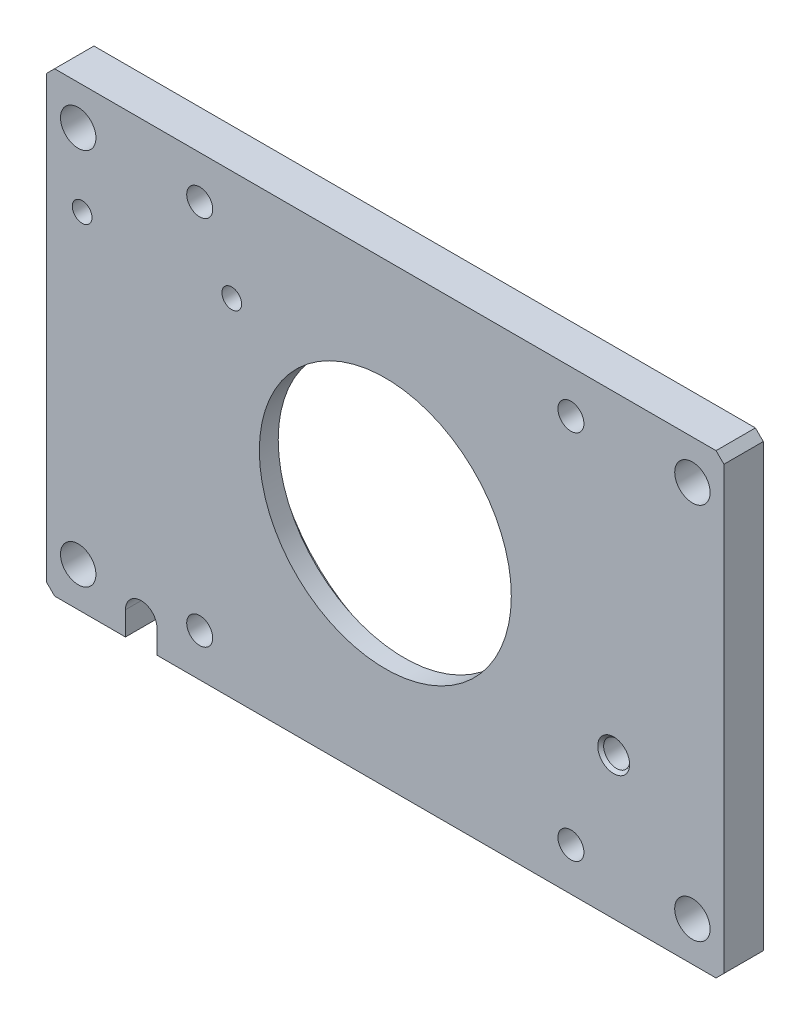
from build123d import *

# Parameters (mm, degrees)
SKETCH_1_W                   = 86
SKETCH_1_H                   = 58
SKETCH_1_R                   = 16
SKETCH_1_R_2                 = 2.25
EXTRUDE_1_DEPTH              = 5
HOLE_WIZARD_M3_1_D           = 2.5
HOLE_WIZARD_M4_1_D           = 3.3
MIRROR_2_COPY_1_D            = 3.3
CUT_EXTRUDE_1_DEPTH          = 53.820450585
CHAMFER_1_SIZE               = 1
SKETCH_10_W                  = 216.550460162
SKETCH_10_H                  = 17.046792279
CUT_EXTRUDE_4_DEPTH          = 73.374028491
SKETCH_11_R                  = 19.5
CUT_EXTRUDE_5_DEPTH          = 2.6
SKETCH_13_R                  = 1.350406535
CUT_EXTRUDE_6_DEPTH          = 10
HOLE_WIZARD_M4_3_D           = 3.3
HOLE_WIZARD_M4_3_DEPTH       = 11.5
HOLE_WIZARD_M4_3_CSINK_D     = 4.05
HOLE_WIZARD_M4_3_CSINK_ANGLE = 90
HOLE_WIZARD_M4_3_TIP         = 0.991420021


with BuildPart() as part:
    # 草图1 → 凸台-拉伸1 (new, symmetric)
    with BuildSketch(Plane.XY):
        Rectangle(SKETCH_1_W, SKETCH_1_H)
        Circle(SKETCH_1_R, mode=Mode.SUBTRACT)
        with Locations((-39, 24)):
            Circle(SKETCH_1_R_2, mode=Mode.SUBTRACT)
        with Locations(Location((39, 24, 0), (0, 0, 180))):
            Circle(SKETCH_1_R_2, mode=Mode.SUBTRACT)
        with Locations((39, -24)):
            Circle(SKETCH_1_R_2, mode=Mode.SUBTRACT)
        with Locations(Location((-39, -24, 0), (0, 0, 180))):
            Circle(SKETCH_1_R_2, mode=Mode.SUBTRACT)
    extrude(amount=EXTRUDE_1_DEPTH, both=True)

    # M3 螺纹孔1 (through all)
    with Locations(Plane.XY.offset(5)):
        with Locations((-38.5, 15), (-19.5, 15)):
            Hole(HOLE_WIZARD_M3_1_D / 2)

    # M4 螺纹孔1 (through all)
    with Locations(Plane.XY.offset(5)):
        with Locations((-23.57, 23.57)):
            hole_wizard_m4_1 = Hole(HOLE_WIZARD_M4_1_D / 2)

    # 镜向1: M4 螺纹孔1 across plane
    add(hole_wizard_m4_1.mirror(Plane.ZX), mode=Mode.SUBTRACT)

    # 镜向2: M4 螺纹孔1 across plane
    add(hole_wizard_m4_1.mirror(Plane(origin=(0, 0, 0), x_dir=(0, 0, 1), z_dir=(1, 0, 0))), mode=Mode.SUBTRACT)

    # 镜向2 copy 1 (through all)
    with Locations(Plane(origin=(0, 0, 5), x_dir=(-1, 0, 0), z_dir=(0, 0, 1))):
        with Locations((-23.57, 23.57)):
            Hole(MIRROR_2_COPY_1_D / 2)

    # 草图7 → 切除-拉伸1 (cut, through all)
    with BuildSketch(Plane.XY.offset(5)):
        with BuildLine():
            Line((-33, -29), (-33, -26))
            ThreePointArc((-33, -26), (-31, -24), (-29, -26))
            Line((-29, -26), (-29, -29))
            ThreePointArc((-29, -29), (-31, -31), (-33, -29))
        make_face()
    extrude(amount=-CUT_EXTRUDE_1_DEPTH, mode=Mode.SUBTRACT)

    # 倒角1
    chamfer_1_edges = [part.edges().sort_by_distance(p)[0] for p in [
        (43, -29, 0),
        (-43, -29, 0),
        (-43, 29, 0),
        (43, 29, 0),
    ]]
    chamfer(chamfer_1_edges, length=CHAMFER_1_SIZE)

    # 草图10 → 切除-拉伸4 (cut, through all)
    with BuildSketch(Plane(origin=(0, 29, 0), x_dir=(1, 0, 0), z_dir=(0, 1, 0))):
        with Locations((51.936518235, 8.52339614)):
            Rectangle(SKETCH_10_W, SKETCH_10_H)
    extrude(amount=-CUT_EXTRUDE_4_DEPTH, mode=Mode.SUBTRACT)

    # 草图11 → 切除-拉伸5 (cut)
    with BuildSketch(Plane(origin=(0, 0, 0), x_dir=(-1, 0, 0), z_dir=(0, 0, -1))):
        Circle(SKETCH_11_R)
    extrude(amount=-CUT_EXTRUDE_5_DEPTH, mode=Mode.SUBTRACT)

    # 草图13 → 切除-拉伸6 (cut)
    with BuildSketch(Plane.XY.offset(5)):
        with Locations((29, -11)):
            Circle(SKETCH_13_R)
    extrude(amount=-CUT_EXTRUDE_6_DEPTH, mode=Mode.SUBTRACT)

    # M4 螺纹孔3
    with Locations(Plane(origin=(29, -11, 5), x_dir=(1, 0, 0), z_dir=(0, 0, 1))):
        with Locations((0, 0)):
            CounterSinkHole(HOLE_WIZARD_M4_3_D / 2, HOLE_WIZARD_M4_3_CSINK_D / 2, depth=HOLE_WIZARD_M4_3_DEPTH, counter_sink_angle=HOLE_WIZARD_M4_3_CSINK_ANGLE)
            with Locations((0, 0, -(HOLE_WIZARD_M4_3_DEPTH + HOLE_WIZARD_M4_3_TIP / 2))):  # 118° drill point
                Cone(0, HOLE_WIZARD_M4_3_D / 2, HOLE_WIZARD_M4_3_TIP, mode=Mode.SUBTRACT)


solid = part.part
